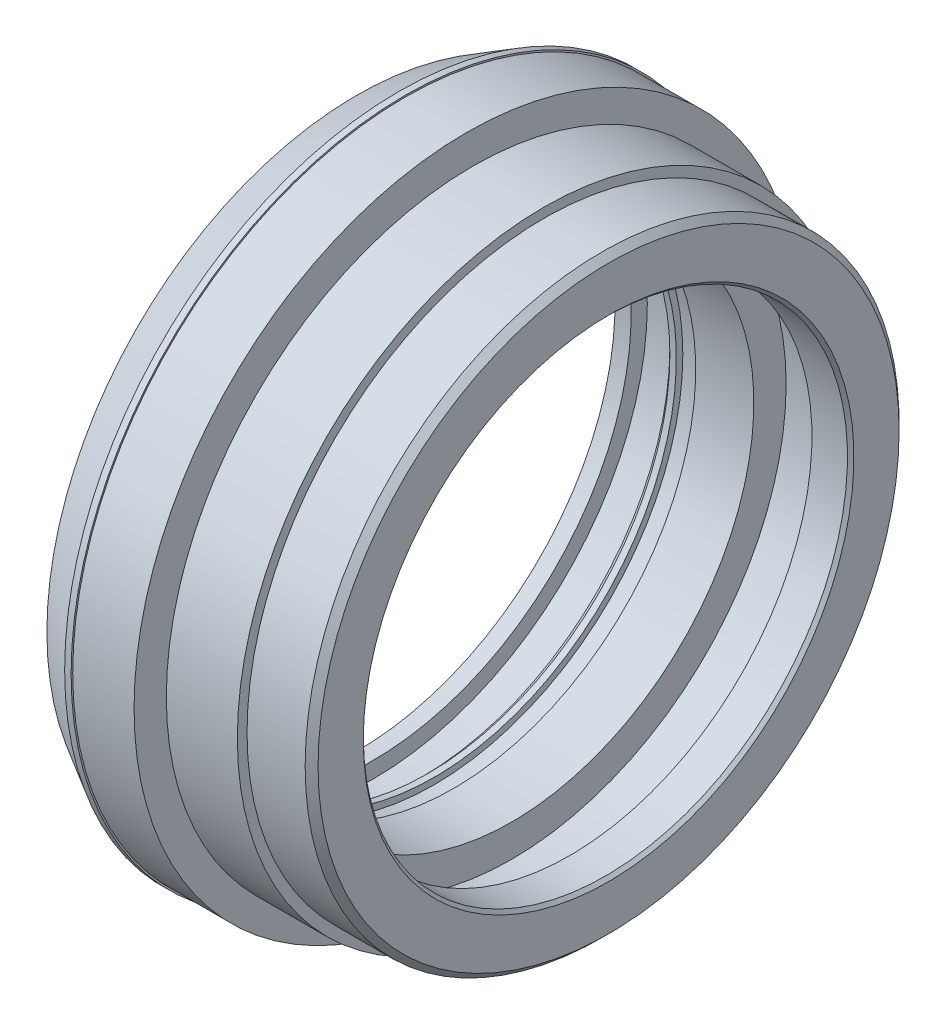
from build123d import *

# Parameters (mm, degrees)
CHAMFER_1_SIZE = 1
CHAMFER_2_SIZE = 0.5
CHAMFER_3_SIZE = 1


with BuildPart() as part:
    # 草图1 → 旋转1 (revolve)
    with BuildSketch(Plane(origin=(0, 0, 0), x_dir=(1, 0, 0), z_dir=(0, 1, 0)), mode=Mode.PRIVATE) as revolve_1_sk:
        Polygon((5.034928566, 40), (7.534928566, 40), (7.534928566, 42.5), (15.034928566, 42.5), (15.034928566, 37.5), (17.034928566, 37.5), (17.034928566, 38.5), (20.034928566, 38.5), (20.034928566, 37.5), (29.034928566, 37.5), (29.034928566, 42.5), (38.034928566, 42.5), (38.034928566, 37.5), (44.034928566, 37.5), (44.034928566, 46), (34.034928566, 46), (34.034928566, 47.5), (23.034928566, 47.5), (23.034928566, 46), (22.034928566, 46), (22.034928566, 51.5), (12.534928566, 51.5), (12.534928566, 51.75), (11.534928566, 51.75), (5.034928566, 48), align=None)
    revolve(revolve_1_sk.sketch.rotate(Axis((-85.103190975, 0, 0), (1, 0, 0)), 180), axis=Axis((-85.103190975, 0, 0), (1, 0, 0)))

    # 倒角1
    chamfer_1_edges = [part.edges().sort_by_distance(p)[0] for p in [
        (44.034928566, 0, -46),
    ]]
    chamfer(chamfer_1_edges, length=CHAMFER_1_SIZE)

    # 倒角2
    chamfer_2_edges = [part.edges().sort_by_distance(p)[0] for p in [
        (44.034928566, 0, -37.5),
    ]]
    chamfer(chamfer_2_edges, length=CHAMFER_2_SIZE)

    # 倒角3
    chamfer_3_edges = [part.edges().sort_by_distance(p)[0] for p in [
        (15.034928566, 0, -37.5),
    ]]
    chamfer(chamfer_3_edges, length=CHAMFER_3_SIZE)


solid = part.part
